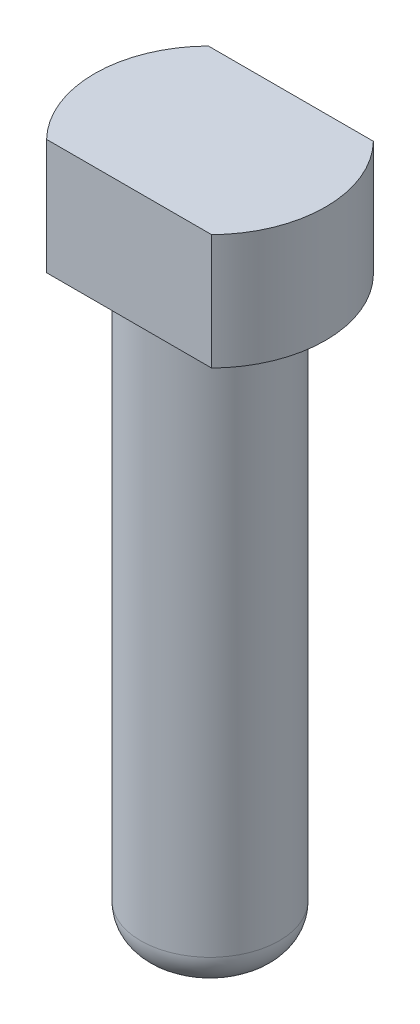
from build123d import *

# Parameters (mm, degrees)
SKETCH_1_R          = 10
EXTRUDE_1_DEPTH     = 30
CUT_EXTRUDE_START   = -50
SKETCH_2_R          = 10
SKETCH_2_R_2        = 6
CUT_EXTRUDE_1_DEPTH = 50
FILLET_1_R          = 3
CUT_EXTRUDE_3_DEPTH = 10


with BuildPart() as part:
    # 草图1 → 凸台-拉伸1 (new, symmetric)
    with BuildSketch(Plane(origin=(0, 0, 0), x_dir=(1, 0, 0), z_dir=(0, 1, 0))):
        with Locations(Location((0, 0, 0), (0, 0, 270))):
            Circle(SKETCH_1_R)
    extrude(amount=EXTRUDE_1_DEPTH, both=True)

    # 草图2 → 切除-拉伸1 (cut)
    with BuildSketch(Plane.XZ.offset(30).offset(CUT_EXTRUDE_START)):
        with Locations(Location((0, 0, 0), (0, 0, 270))):
            Circle(SKETCH_2_R)
        with Locations(Location((0, 0, 0), (0, 0, 270))):
            Circle(SKETCH_2_R_2, mode=Mode.SUBTRACT)
    extrude(amount=CUT_EXTRUDE_1_DEPTH, mode=Mode.SUBTRACT)

    # 圆角1
    fillet_1_edges = [part.edges().sort_by_distance(p)[0] for p in [
        (0, -30, 6),
    ]]
    fillet(fillet_1_edges, radius=FILLET_1_R)

    # 草图3 → 切除-拉伸3 (cut)
    with BuildSketch(Plane(origin=(0, 30, 0), x_dir=(1, 0, 0), z_dir=(0, 1, 0))):
        with BuildLine():
            Line((-7.141428429, 7), (7.141428429, 7))
            ThreePointArc((7.141428429, 7), (0, 10), (-7.141428429, 7))
        make_face()
        with BuildLine():
            Line((-7.141428429, -7), (7.141428429, -7))
            ThreePointArc((7.141428429, -7), (0, -10), (-7.141428429, -7))
        make_face()
    extrude(amount=-CUT_EXTRUDE_3_DEPTH, mode=Mode.SUBTRACT)


solid = part.part
